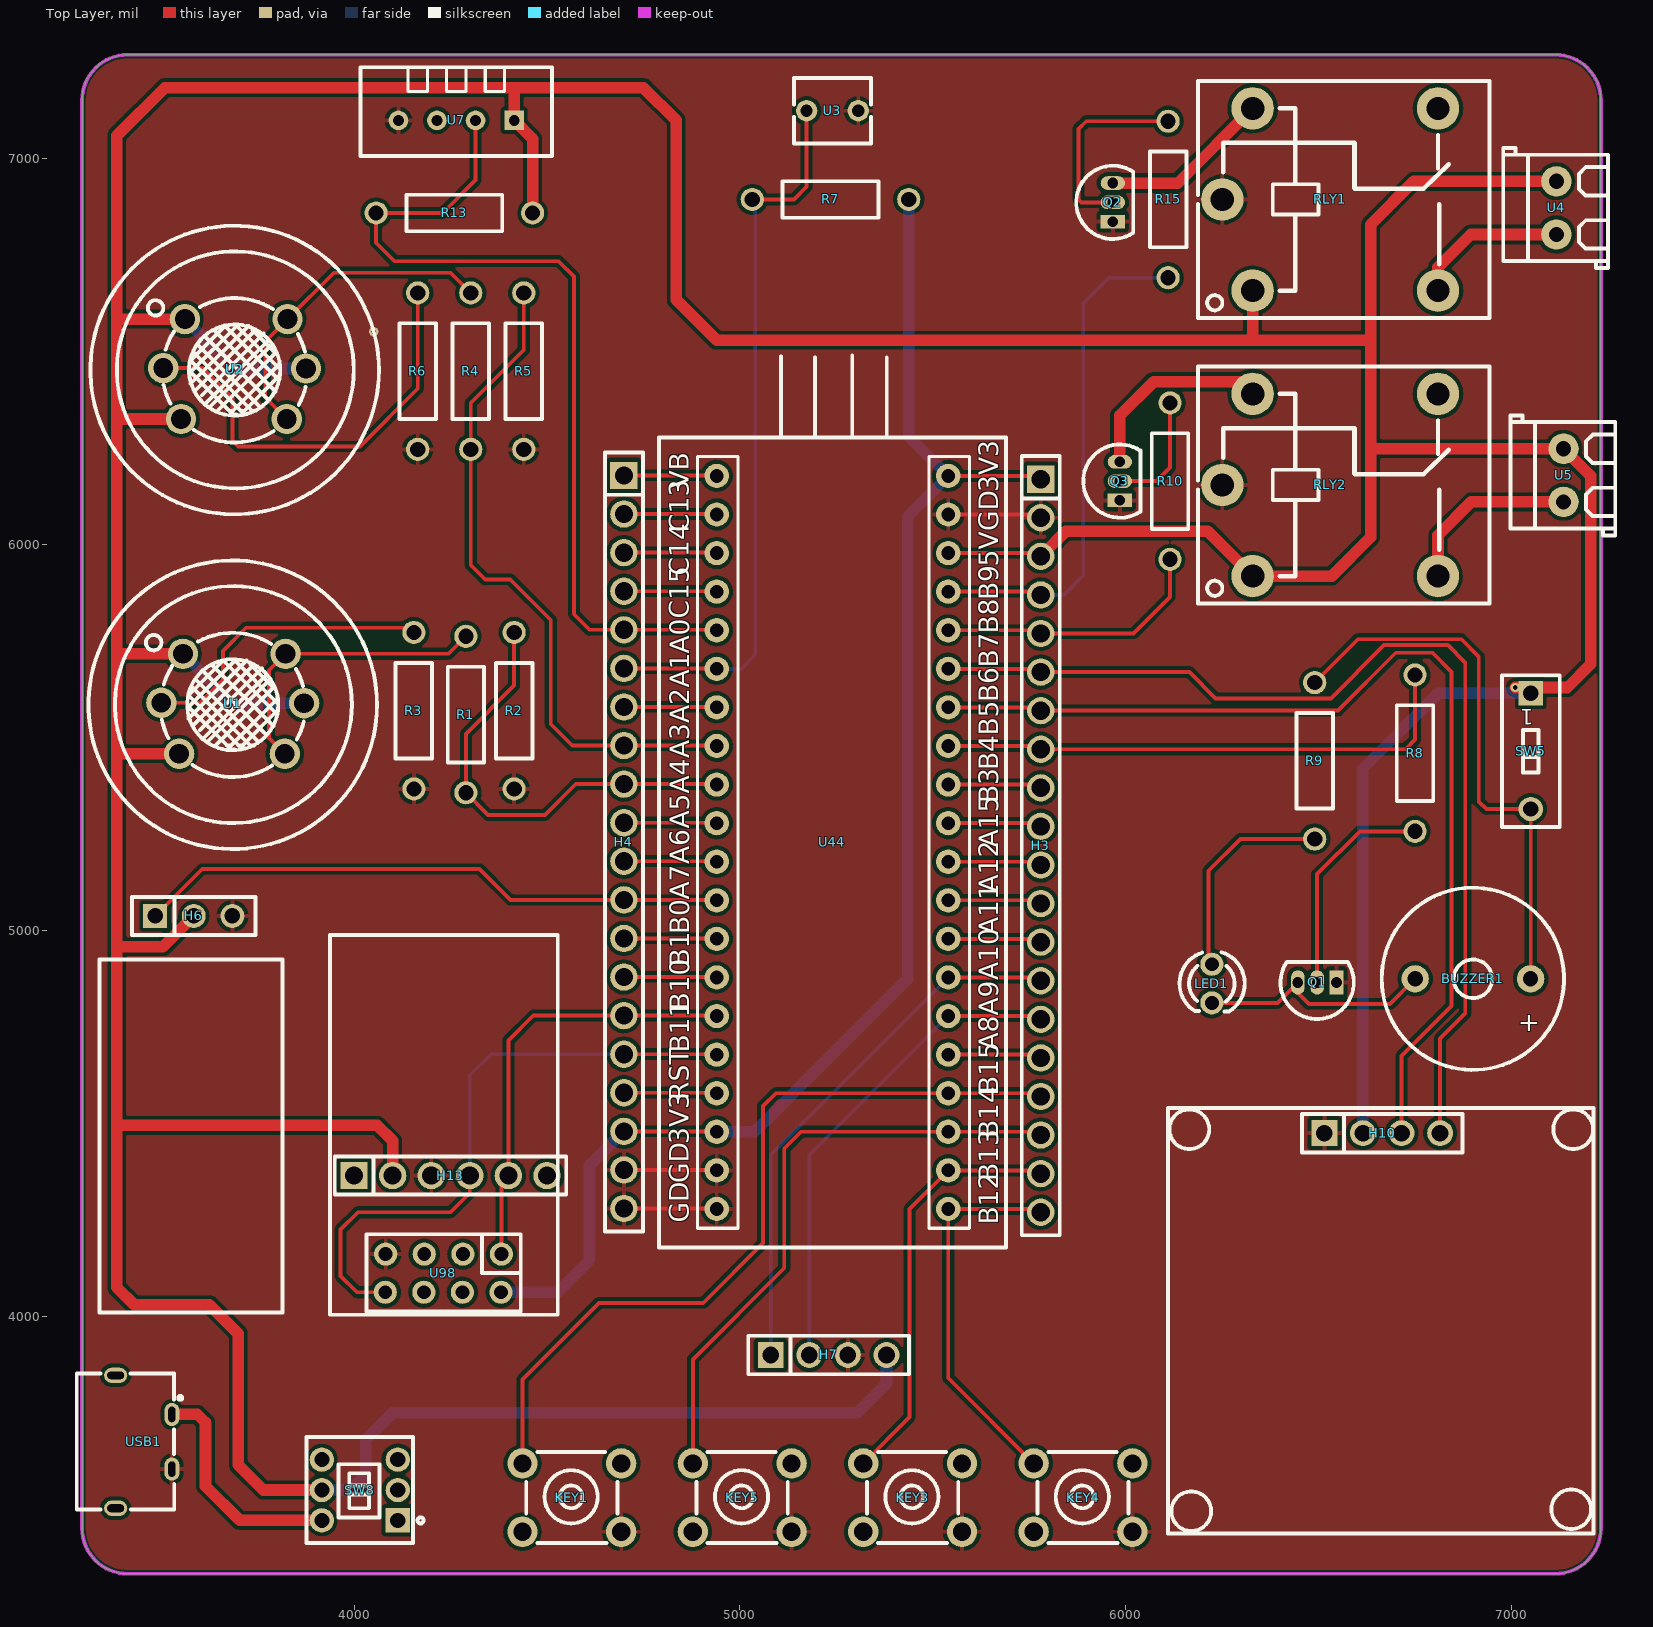
[diagram p0: Top Layer view]
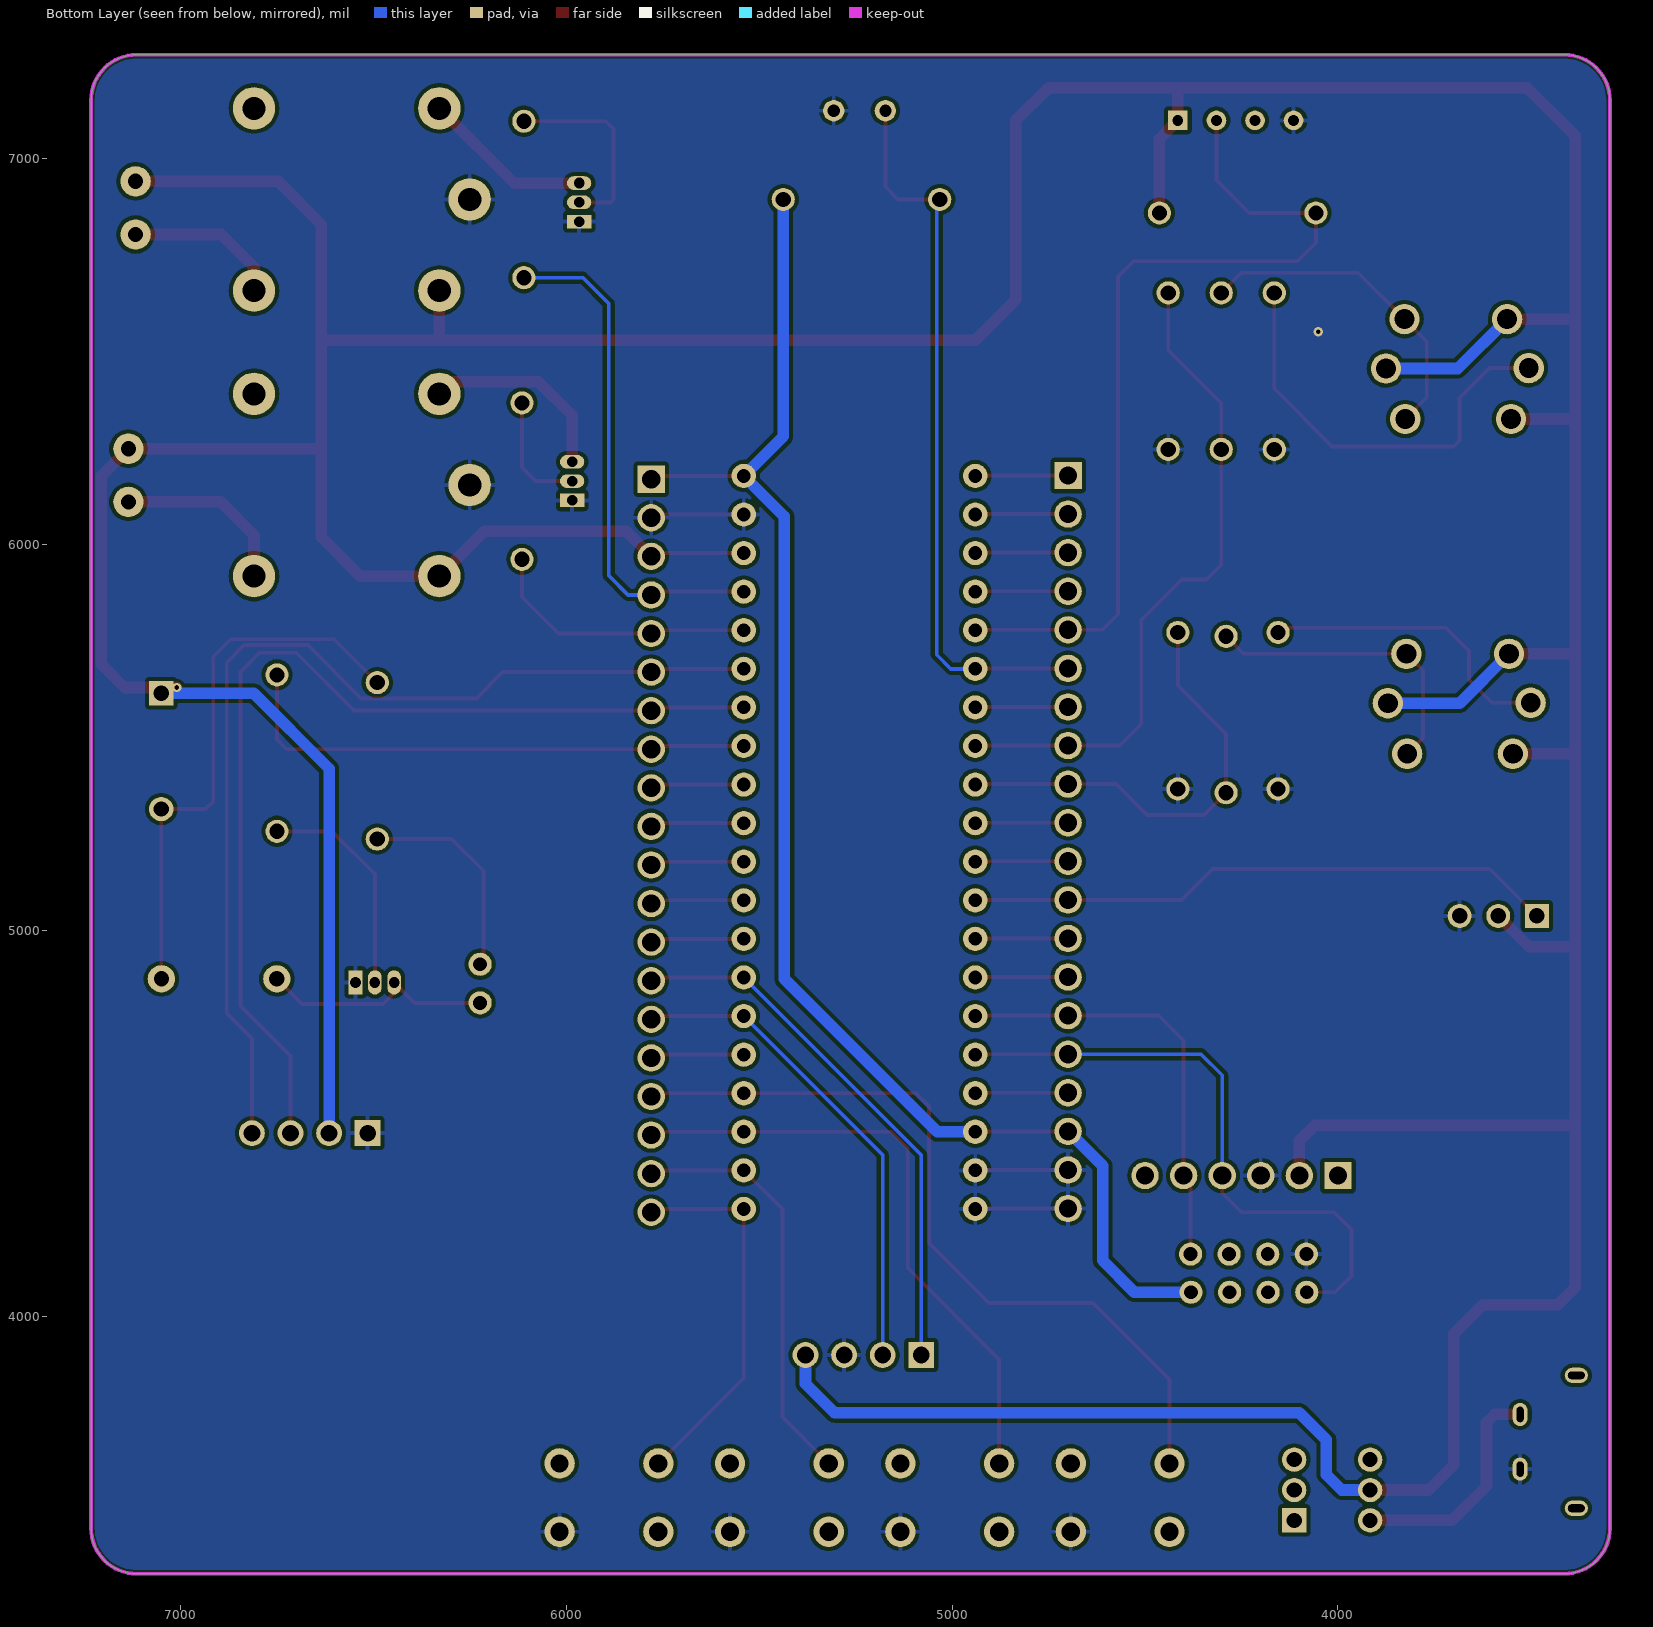
[diagram p1: Bottom Layer view, seen from below]
# Altium PCB MISC62290.pcbdoc
Units mil, origin at the board's own origin, x right, y up, seen from the top; angles counter-clockwise.
Board outline 3937.01 x 3937.01 mil, 2 copper layers (Top Layer, Bottom Layer), stack 62.206 mil thick; 40 components, 52 nets, 202 pads, 2 vias.

## Layer stack, top to bottom
Top Solder Mask Layer: solder mask 0.394, Dk 3.3
Top Layer: signal copper 1.379
Dielectric1: surface 59.449, FR4, Dk 4.5
Bottom Layer: signal copper 1.378
Bottom Solder Mask Layer: solder mask 0.394, Dk 3.3

## Board outline
3413.11,7270 ccw(c3413.11,7151.89) 3295,7151.89 3295,3451.1 ccw(c3413.11,3451.1) 3413.11,3332.99 7113.9,3332.99 ccw(c7113.9,3451.1) 7232.01,3451.1 7232.01,7151.89 ccw(c7113.9,7151.89) 7113.9,7270

## Design rules (kind name [scope] priority, off if disabled: settings)
BoardOutlineClearance copperThickness2oz_1 [All] p2 off: genericclearance=7.99 ignorepadtopadclearanceinfootprint=FALSE except(0: Arc-SplitContinuation Track-SplitContinuation SMDPad-SplitContinuation THPad-SplitContinuation Via-SplitContinuation Fill-SplitContinuation Region-SplitContinuation Poly-SplitContinuation Text-SplitContinuation Hole-SplitContinuation; 5.98: Arc-CutoutEdge SMDPad-CutoutEdge THPad-CutoutEdge Via-CutoutEdge Fill-CutoutEdge Region-CutoutEdge Text-CutoutEdge; 6.93: Hole-OutlineEdge Hole-CutoutEdge; 10: Poly-OutlineEdge Poly-CutoutEdge; 11.81: Arc-OutlineEdge Track-OutlineEdge SMDPad-OutlineEdge THPad-OutlineEdge Via-OutlineEdge Fill-OutlineEdge Region-OutlineEdge Text-OutlineEdge Track-CutoutEdge)
BoardOutlineClearance copperThickness1oz_1 [All] p4: genericclearance=4.02 ignorepadtopadclearanceinfootprint=FALSE except(0: Arc-SplitContinuation Track-SplitContinuation SMDPad-SplitContinuation THPad-SplitContinuation Via-SplitContinuation Fill-SplitContinuation Region-SplitContinuation Poly-SplitContinuation Text-SplitContinuation Hole-SplitContinuation; 6: SMDPad-CutoutEdge THPad-CutoutEdge Via-CutoutEdge Fill-CutoutEdge Region-CutoutEdge Text-CutoutEdge; 6.93: Hole-OutlineEdge Hole-CutoutEdge; 10: Poly-OutlineEdge Poly-CutoutEdge; 11.8: Arc-OutlineEdge Track-OutlineEdge SMDPad-OutlineEdge THPad-OutlineEdge Via-OutlineEdge Fill-OutlineEdge Region-OutlineEdge Text-OutlineEdge; 11.81: Arc-CutoutEdge Track-CutoutEdge)
Clearance copperThickness2oz [All] p1 off: gap=7.99 ignorepadtopadclearanceinfootprint=FALSE except(5.98: SMDPad-Track SMDPad-SMDPad THPad-Track SMDPad-THPad THPad-THPad Track-Via SMDPad-Via THPad-Via Via-Via Fill-Track Region-Track Fill-SMDPad Region-SMDPad Fill-THPad Region-THPad Fill-Via Region-Via Fill-Fill Fill-Region Region-Region Arc-Track Arc-SMDPad Arc-THPad Arc-Via Fill-Arc Region-Arc Arc-Arc Text-Track SMDPad-Text Text-THPad Text-Via Fill-Text Region-Text Arc-Text Text-Text; 6.93: Hole-Track Hole-SMDPad Hole-THPad Hole-Via Fill-Hole Region-Hole Hole-Arc Hole-Text; 10: Poly-Track Poly-SMDPad Poly-THPad Poly-Via Poly-Fill Poly-Region Poly-Poly Poly-Arc Poly-Text Poly-Hole)
Clearance copperThickness1oz [All] p3: gap=4.02 ignorepadtopadclearanceinfootprint=FALSE except(5.98: SMDPad-Track SMDPad-SMDPad THPad-Track SMDPad-THPad THPad-THPad Track-Via SMDPad-Via THPad-Via Via-Via Fill-Track Region-Track Fill-SMDPad Region-SMDPad Fill-THPad Region-THPad Fill-Via Region-Via Fill-Fill Fill-Region Region-Region; 6: Arc-Track Arc-SMDPad Arc-THPad Arc-Via Fill-Arc Region-Arc Arc-Arc Text-Track SMDPad-Text Text-THPad Text-Via Fill-Text Region-Text Arc-Text Text-Text; 6.93: Hole-Track Hole-SMDPad Hole-THPad Hole-Via Fill-Hole Region-Hole Hole-Arc Hole-Text; 10: Poly-Track Poly-SMDPad Poly-THPad Poly-Via Poly-Fill Poly-Region Poly-Poly Poly-Arc Poly-Text Poly-Hole)
Creepage creepage [All] p1: checkdistance=0 ignoreinternallayers=TRUE applytopolygonpour=TRUE
DiffPairsRouting differentialPair [All] p1: maxlimit=6 minlimit=6 mostfreqgap=6 toplayer_minwidth=5 toplayer_prefwidth=10 toplayer_maxwidth=100 toplayer_mingap=6 toplayer_prefgap=6 toplayer_maxgap=6 bottomlayer_minwidth=5 bottomlayer_prefwidth=10 bottomlayer_maxwidth=100 bottomlayer_mingap=6 bottomlayer_prefgap=6 bottomlayer_maxgap=6 maxuncoupledlength=10
HoleToHoleClearance otherClearance [All] p1: gap=11.81 allowstackedmicrovias=TRUE
Length netLength [All] p1: minlimit=0 maxlimit=0
MatchedLengths netLengthTolerance [All] p1: tolerance=1000
PasteMaskExpansion pasteMaskExpansion [All] p1: expansion=0
PlaneConnect innerPlane [All] p1: planeconnectstyle=Relief reliefexpansion=20 reliefentries=4 reliefconductorwidth=10 reliefairgap=10
PolygonConnect copperRegion [(InNet('GND'))] p1: connectstyle=Relief reliefconductorwidth=10 reliefentries=4 polygonreliefangle="90 Angle" airgapwidth=10 via.connectstyle=Relief via.reliefconductorwidth=10 via.reliefentries=4 via.polygonreliefangle="90 Angle" via.airgapwidth=10
RoutingVias viaSize [All] p1: holewidth=12.01 width=24.02 viastyle="Through Hole" minholewidth=11.81 minwidth=19.68 maxholewidth=248.03 maxwidth=393.7
SolderMaskExpansion solderMaskExpansion [IsVia] p1: expansion=-1000 istentingtop=TRUE
SolderMaskExpansion solderMaskExpansion [All] p2: expansion=2 istentingtop=FALSE
Width copperThickness2oz_2 [All] p1 off: maxlimit=100 minlimit=8 preferedwidth=10
Width copperThickness1oz_2 [All] p2: maxlimit=100 minlimit=5 preferedwidth=10

## Components (designator, comment, footprint, x,y, rotation, side; value= is the part's Value field where it differs from the comment)
BUZZER1 "2.3kHz" BUZ-TH_BD12.0-P7.60-D0.6-FD 6900,4875 r180 top
H3 "" HDR-TH_20P-P2.54-V-F 5780,5220 r270 top
H4 "" HDR-TH_20P-P2.54-V-F 4699.46,5229.58 r270 top
H6 "" HDR-TH_3P-P2.54-V-F 3584.58,5037.88 r0 top
H7 "" HDR-TH_4P-P2.54-V-F 5230,3900 r0 top
H10 "2.54-1*4P female" HDR-TH_4P-P2.54-V-F 6665,4475 r0 top
H13 "" HDR-TH_6P-P2.54-V-M-1 4250,4365 r0 top
KEY1 "Button 1" KEY-TH_4P-L6.0-W6.0-P4.50-LS7.5 4564.46,3530.41 r0 top
KEY3 "Button 2" KEY-TH_4P-L6.0-W6.0-P4.50-LS7.5 5447.8,3530.41 r0 top
KEY4 "Button 4" KEY-TH_4P-L6.0-W6.0-P4.50-LS7.5 5889.46,3530.41 r0 top
KEY5 "Button 5" KEY-TH_4P-L6.0-W6.0-P4.50-LS7.5 5006.13,3530.41 r0 top
LED1 "" LED_TH-3mm 6223.5,4862.73 r270 top
Q1 "" S8050_TO_92 6496.32,4865.58 r180 top
Q2 "" S8050_TO_92 5966.77,6887.54 r90 top
Q3 "" S8050_TO_92 5985,6165 r90 top
R1 "10kΩ" Res_1/4W 4290,5560 r90 top
R2 "10kΩ" Res_1/4W 4415,5570 r90 top
R3 "5Ω" Res_1/4W 4155,5570 r90 top
R4 "10kΩ" Res_1/4W 4302.5,6450 r90 top
R5 "10kΩ" Res_1/4W 4440,6450 r90 top
R6 "5Ω" Res_1/4W 4165,6450 r90 top
R7 "1kΩ" Res_1/4W 5235,6895 r180 top
R8 "1kΩ" Res_1/4W 6750,5460 r270 top
R9 "120" Res_1/4W 6490,5440 r270 top
R10 "1kΩ" Res_1/4W 6115,6165 r90 top
R13 "10kΩ" Res_1/4W 4260,6860 r0 top
R15 "1kΩ" Res_1/4W 6110,6895 r90 top
RLY1 "SRD-05VDC-SL-C" RELAY-TH_SRD-XXVDC-XL-C 6530,6895 r0 top
RLY2 "SRD-05VDC-SL-C" RELAY-TH_SRD-XXVDC-XL-C 6530,6155 r0 top
SW5 "NDS-01V" SW-TH_2P-L3.9-W9.9-P2.54-LS7.6 7050,5465 r270 top
SW8 "TK-6700-1" SW-TH_TK-6700-1 4015,3550 r90 top
U1 "MQ-2" SENSOR-TH_MQ-2 3685.58,5587.88 r0 top
U2 "MQ-5" SENSOR-TH_MQ-2 3690.58,6455.41 r0 top
U3 "光敏电阻-5MM" RES-TH_L4.9-W4.3-P3.4 5240,7125 r180 top
U4 "KF350-3.5-2P" CONN-TH_P3.50_KF350-3.5-2P 7116.51,6873.11 r90 top
U5 "KF350-3.5-2P" CONN-TH_P3.50_KF350-3.5-2P 7135,6180 r90 top
U7 "DHT11" SENSOR-TH_DHT11 4265,7100 r180 top
U44 "" STM32最小系统板 5280,5485 r0 top
U98 "" WiFi封装 4230,4370 r0 top
USB1 "KH-TYPE-C-2P" USB-SMD_KH-TYPE-C-2P 3455,3675 r270 top

## Footprints (in the part's own frame and the unit in brackets; to place one, negate y for a bottom-side part, rotate by r counter-clockwise, add the part's x,y. Pads: shape width x height; smd on the part's side, far side on the other; paste and mask are expansions set on the pad)
BUZ-TH_BD12.0-P7.60-D0.6-FD [mm]
  round 1.8 hole 1 paste+0 mask+0.051: 1(-3.8,0) 2(3.8,0)
  silkscreen extent -6,-6 6,6
CONN-TH_P3.50_KF350-3.5-2P [mm]
  round 2 hole 1: 1(-1.75,0) 2(1.75,0)
  silkscreen extent -3.95,-3.4 3.95,3.5
HDR-TH_3P-P2.54-V-F [mil]
  rect 62x62 hole 40.16: 1(-100,0)
  round 62 hole 40.16: 2(0,0) 3(100,0)
  silkscreen extent -160,-49 160,49
HDR-TH_4P-P2.54-V-F [mm]
  rect 1.7x1.7 hole 1.1: 1(-3.81,0)
  round 1.7 hole 1.1: 2(-1.27,0) 3(1.27,0) 4(3.81,0)
  silkscreen extent -5.29,-1.27 5.29,1.27
HDR-TH_6P-P2.54-V-M-1 [mm]
  rect 1.8x1.8 hole 1.2: 1(-6.35,0)
  round 1.8 hole 1.2: 2(-3.81,0) 3(-1.27,0) 4(1.27,0) 5(3.81,0) 6(6.35,0)
  silkscreen extent -7.62,-1.25 7.62,1.25
HDR-TH_20P-P2.54-V-F [mm]
  rect 1.8x1.8 hole 1.2: 1(-24.13,0)
  round 1.8 hole 1.2: 2(-21.59,0) 3(-19.05,0) 4(-16.51,0) 5(-13.97,0) 6(-11.43,0) 7(-8.89,0) 8(-6.35,0) 9(-3.81,0) 10(-1.27,0) 11(1.27,0) 12(3.81,0) 13(6.35,0) 14(8.89,0) 15(11.43,0) 16(13.97,0) 17(16.51,0) 18(19.05,0) 19(21.59,0) 20(24.13,0)
  silkscreen extent -25.65,-1.25 25.65,1.25
KEY-TH_4P-L6.0-W6.0-P4.50-LS7.5 [mm]
  round 2 hole 1.2 paste+0 mask+0.051: 1(-3.25,-2.25) 2(3.25,-2.25) 3(3.25,2.25) 4(-3.25,2.25)
  silkscreen extent -3,-3 3,3
LED_TH-3mm [mil]
  round 60 hole 36 paste+0 mask+2: 1(-50,0) 2(50,0)
  silkscreen extent -81,-84 72,85
RELAY-TH_SRD-XXVDC-XL-C [mil]
  round 110 hole 60: 1(-200.79,-236.22) 2(279.52,-236.2) 3(279.53,236.2) 4(-200.79,236.22) 5(-279.53,0)
  silkscreen extent -342,-307 413,307
RES-TH_L4.9-W4.3-P3.4 [mm]
  round 1.4 hole 0.8 paste+0 mask+0.05: 1(-1.7,0) 2(1.7,0)
  silkscreen extent -2.54,-2.16 2.54,2.16
Res_1/4W [mil]
  round 60 hole 39.37 paste+0 mask+2: 1(-202.76,0) 2(202.76,0)
  silkscreen extent -124,-47 124,47
S8050_TO_92 [mil]
  rect 35.4x63 hole 27.6 paste+0 mask+2: 1(-50,0)
  oval 35.4x63 hole 27.6 paste+0 mask+2: 2(0,0) 3(50,0)
  silkscreen extent -95,-53 95,95
SENSOR-TH_DHT11 [mil]
  rect 51x51 hole 28: 1(-150,0)
  round 51 hole 28: 2(-50,0) 3(50,0) 4(150,0)
  silkscreen extent -248,-138 248,93
SENSOR-TH_MQ-2 [mil]
  round 78.74 hole 51.18: 1(-129,129.5) 2(-185,2.5) 3(-139,-129.5) 4(135,-129.5) 5(185,1.5) 6(137,129.5)
  silkscreen extent -374,-376 374,371
STM32最小系统板 [mm]
  round 1.6 hole 0.9: 1(-8.634,17.614) 2(-8.634,15.074) 3(-8.634,12.534) 4(-8.634,9.994) 5(-8.634,7.454) 6(-8.634,4.914) 7(-8.634,2.374) 8(-8.634,-0.166) 9(-8.634,-2.706) 10(-8.634,-5.246) 11(-8.634,-7.786) 12(-8.634,-10.326) 13(-8.634,-12.866) 14(-8.634,-15.406) 15(-8.634,-17.946) 16(-8.634,-20.486) 17(-8.634,-23.026) 18(-8.634,-25.566) 19(-8.634,-28.106) 20(-8.634,-30.646) 21(6.606,17.614) 22(6.606,15.074) 23(6.606,12.534) 24(6.606,9.994) 25(6.606,7.454) 26(6.606,4.914) 27(6.606,2.374) 28(6.606,-0.166) 29(6.606,-2.706) 30(6.606,-5.246) 31(6.606,-7.786) 32(6.606,-10.326) 33(6.606,-12.866) 34(6.606,-15.406) 35(6.606,-17.946) 36(6.606,-20.486) 37(6.606,-23.026) 38(6.606,-25.566) 39(6.606,-28.106) 40(6.606,-30.646)
  silkscreen extent -12.44,-33.19 10.42,25.54
SW-TH_2P-L3.9-W9.9-P2.54-LS7.6 [mm]
  rect 1.6x1.6 hole 1 paste+0 mask+0.05: 1(-3.81,0)
  round 1.6 hole 1 paste+0 mask+0.05: 2(3.81,0)
  silkscreen extent -5,-1.91 5,1.91
SW-TH_TK-6700-1 [mm]
  rect 1.6x1.6 hole 1 paste+0 mask+0.051: 1(-2,-2.5)
  round 1.6 hole 1 paste+0 mask+0.051: 2(0,-2.5) 3(2,-2.5)
  round 1.6 hole 1 copper offset 0,0 paste+0 mask+0.051: 4(-2,2.5) 5(0,2.5) 6(2,2.5)
  silkscreen extent -3.5,-4.2 3.5,3.5
USB-SMD_KH-TYPE-C-2P [mm]
  oval 1.524x1 hole 0.45 slot 1 at 0 deg paste+0 mask+0.05: 1(-1.8,1.85) 2(1.8,1.85)
  oval 1x1.524 hole 0.5 slot 1.1 at 90 deg paste+0 mask+0.05: 3(4.375,-1.85) 4(-4.375,-1.85)
  silkscreen extent -4.5,-4.41 4.46,2.53
WiFi封装 [mil]
  round 60 hole 36: 1(152.01,-208.54) 2(150.91,-307.4) 3(52.01,-208.54) 4(50.91,-307.4) 5(-47.99,-208.54) 6(-49.09,-307.4) 7(-147.99,-208.54) 8(-149.09,-307.4)
  silkscreen extent -293,-366 298,618

## Via types
v1: diameter 24.02, hole 12, Top Layer to Bottom Layer, 2 vias

## Nets (pads, with @x,y where several pads share a name; then routed paths per layer and width w, separated by ;. In a path a pad name is that pad's centre, name@x,y a point inside that pad or via, vN(x,y) a via of type N, cw(c..) or ccw(c..) an arc to the next point about the centre after c; other vN are vias at no path point)
3V3: H3.1 H4.18 R7.1 U44.18 U44.21 U98.2 | length 3895.4
  Top Layer w10: H4.18 U44.18@4940,4479.58 ; U44.21 H3.1@5795,6178.46
  Bottom Layer w30: U98.2 4527.6,4062.6 4610,4145 4610,4390.12 H4.18 ; U44.18 5038.46,4478.46 5435,4875 5435,6073.39 U44.21 5437.76,6280.78 R7.1
$1N3: R1.2 U1.4 U1.6 | length 779.7
  Top Layer w10: U1.4 3780,5498.95 3780,5674.8 U1.6 4244.61,5717.38 R1.2
$1N5: R3.2 U1.2 | length 784
  Top Layer w10: U1.2 3600.38,5590.38 3660,5650 3660,5725 3720,5785 4142.76,5785 R3.2
$1N8: R6.2 U2.2 | length 1117.8
  Top Layer w10: U2.2 3607.09,6457.91 3685,6380 3685,6270 3700,6255 4015,6255 4165,6405 R6.2
$1N10: R4.2 U2.4 U2.6 | length 852.2
  Top Layer w10: U2.4 3770,6381.49 3770,6527.33 U2.6 3947.67,6705 4250.26,6705 R4.2
$1N88: BUZZER1.1 R9.1 SW5.2 | length 1448.6
  Top Layer w10: R9.1 6602.24,5755 6870,5755 6915,5710 6915,5335 6935,5315 SW5.2 7050,4875.4 BUZZER1.1
$1N89: BUZZER1.2 LED1.2 Q1.3 | length 614.5
  Top Layer w10: LED1.2 6393.47,4812.73 Q1.3 6446.32,4838.68 6475,4810 6685.4,4810 BUZZER1.2
$1N100: H4.17 U44.17 | length 240.5
  Top Layer w10: H4.17 U44.17@4940,4579.58
$1N103: H4.14 U44.14 | length 240.5
  Top Layer w10: H4.14 U44.14@4940,4879.58
$1N104: H4.13 U44.13 | length 240.5
  Top Layer w10: H4.13 U44.13@4940,4979.58
$1N106: H4.11 U44.11 | length 240.5
  Top Layer w10: H4.11 U44.11@4940,5179.58
$1N110: H4.7 U44.7 | length 240.5
  Top Layer w10: H4.7 U44.7@4940,5579.58
$1N113: H4.4 U44.4 | length 240.5
  Top Layer w10: H4.4 U44.4@4940,5879.58
$1N114: H4.3 U44.3 | length 240.5
  Top Layer w10: H4.3 U44.3@4940,5979.58
$1N115: H4.2 U44.2 | length 240.5
  Top Layer w10: H4.2 U44.2@4940,6079.58
$1N116: H4.1 U44.1 | length 240.5
  Top Layer w10: H4.1 U44.1@4940,6179.58
$1N125: H3.9 U44.29 | length 254.9
  Top Layer w10: U44.29 H3.9@5795,5378.46
$1N126: H3.10 U44.30 | length 254.9
  Top Layer w10: U44.30 H3.10@5795,5278.46
$1N127: H3.11 U44.31 | length 254.9
  Top Layer w10: U44.31 H3.11@5795,5178.46
$1N128: H3.12 U44.32 | length 254.9
  Top Layer w10: U44.32 H3.12@5795,5078.46
$1N129: H3.13 U44.33 | length 254.9
  Top Layer w10: U44.33 H3.13@5795,4978.46
$1N132: H3.16 U44.36 | length 254.9
  Top Layer w10: U44.36 H3.16@5795,4678.46
$1N154: RLY1.2 U4.1 | length 402.8
  Top Layer w30: RLY1.2 6809.53,6719.53 6894.21,6804.21 U4.1
$1N275: Q1.2 R8.2 | length 580.4
  Top Layer w10: Q1.2 6496.32,5146.32 6607.24,5257.24 R8.2
$1N288: Q2.2 R15.2 | length 515.4
  Top Layer w10: Q2.2 5885,6887.54 5877.93,6894.61 5877.93,7077.93 5897.76,7097.76 R15.2
$1N290: Q2.3 RLY1.4 | length 442.7
  Top Layer w30: Q2.3 6135.53,6937.54 RLY1.4
$1N291: Q3.3 RLY2.4 | length 513.6
  Top Layer w30: Q3.3 5985,6335.21 6072.38,6422.59 6297.84,6422.59 RLY2.4
$1N293: Q3.2 R10.2 | length 312.3
  Top Layer w10: Q3.2 6080,6165 6115,6200 R10.2
$1N298: RLY2.2 U5.1 | length 467.1
  Top Layer w30: RLY2.2 6809.53,6024.53 6896.1,6111.1 U5.1
$1N299: LED1.1 R9.2 | length 554.9
  Top Layer w10: LED1.1 6215,4921.24 6215,5155 6297.24,5237.24 R9.2
+5V: H3.3 H6.2 H7.4 H10.2 H13.2 R13.2 RLY1.1 RLY2.1 SW5.1 SW8.5 U1.1 U1.3 U1.5 U2.1 U2.3 U2.5 U4.2 U5.2 U7.1 U44.23 | length 17757.5
  Top Layer w10: U44.23 H3.3@5788.46,5978.46
  Top Layer w30: 3385.03,5717.38 U1.1 ; U1.3 3388.56,5458.38 3385,5461.93 ; U2.3 3388.18,6325.91 3385,6329.09 ; U2.1 3387.29,6584.91 3385,6587.2 ; H6.2 3504.66,4957.95 3385,4957.95 ; SW8.5 3765,3550 3700,3615 3700,3955 3625,4030 3430,4030 3385,4075 3385,4490.1 ; H13.2 4100,4455 4060,4495 3389.9,4495 3385,4490.1 ; R13.2 4462.76,7052.24 U7.1 4415,7183.35 4416.65,7185 ; H3.3 5788.46,5978.46 5845,6035 6212.99,6035 RLY2.1 6533.78,5918.78 6635,6020 6635,6254.11 ; RLY1.1 6329.21,6530.46 6328.75,6530 ; v1(7010,5630) 7145,5630 7205,5690 7205,6178.9 U5.2 6640.22,6248.9 6635,6254.11 ; U4.2 6747,6942 6635,6830 6635,6530 ; 3385,4490.1 3385,4957.95 ; 3385,4957.95 3385,5461.93 ; 3385,5461.93 3385,5717.41 3385,6329.09 ; 3385,6329.09 3385,6587.2 ; 3385,6587.2 3385,7060 3510,7185 4416.65,7185 ; 4416.65,7185 4750,7185 4835,7100 4835,6635 4940,6530 6328.75,6530 ; 6328.75,6530 6635,6530 ; 6635,6254.11 6635,6530
  Bottom Layer w30: U1.1 3684.58,5589.38 U1.5 ; U2.1 3689.58,6456.91 U2.5 ; SW8.5 3990,3550 4030,3590 4030,3680 4100,3750 5305,3750 5380,3825 H7.4 ; H10.2 6615,5420 6810,5615 SW5.1
GND: H3.2 H4.19 H4.20 H6.3 H7.3 H10.1 H13.3 KEY1.2 KEY3.2 KEY4.2 KEY5.2 Q1.1 Q2.1 Q3.1 R2.1 R3.1 R5.1 R6.1 RLY1.5 RLY2.5 U3.1 U7.4 U44.19 U44.20 U44.22 U98.7 USB1.2 | length 736
  Top Layer w10: H4.20 U44.20@4940,4279.58 ; H4.19 U44.19@4940,4379.58 ; U44.22 H3.2@5795,6078.46
  other v1: 4051.2,6552.12
PA0: H4.5 R13.1 U7.2 U44.5 | length 2336.1
  Top Layer w10: U7.2 4315,6945 4230,6860 R13.1 4057.24,6782.76 4105,6735 4530,6735 4570,6695 4570,5820 4610.42,5779.58 H4.5 U44.5@4940,5779.58
PA1: H4.6 R7.2 U3.2 U44.6 | length 1890.3
  Top Layer w10: H4.6 U44.6@4940,5679.58 ; R7.2 5140,6895 5173.07,6928.07 U3.2
  Bottom Layer w10: U44.6 5003.46,5678.46 5040,5715 5040,6887.24 R7.2
PA3: H4.8 R4.1 R5.2 U44.8 | length 1751.7
  Top Layer w10: R5.2 4440,6505 4302.5,6367.5 R4.1 4302.5,5947.5 4340,5910 4405,5910 4510,5805 4510,5535 4565.42,5479.58 H4.8 U44.8@4940,5479.58
PA4: H4.9 R1.1 R2.2 U44.9 | length 1174
  Top Layer w10: R2.2 4415,5635 4290,5510 R1.1 4347.24,5300 4495,5300 4574.58,5379.58 H4.9 U44.9@4940,5379.58
PA5: H4.10 U44.10 | length 240.5
  Top Layer w10: H4.10 U44.10@4940,5279.58
PA7: H4.12 H6.1 U44.12 | length 1539.3
  Top Layer w10: H6.1 3606.7,5160 4325,5160 4405.42,5079.58 H4.12 U44.12@4940,5079.58
PB5: H3.8 R8.1 U44.28 | length 1403
  Top Layer w10: U44.28 H3.8@5795,5478.46 ; H3.8 6725,5470 6750,5495 R8.1
PB6: H3.7 H10.3 U44.27 | length 2651.6
  Top Layer w10: U44.27 H3.7@5795,5578.46 ; H3.7 6550,5570 6700,5720 6795,5720 6845,5670 6845,4805 6715,4675 H10.3
PB7: H3.6 H10.4 U44.26 | length 2706
  Top Layer w10: U44.26 H3.6@5795,5678.46 ; H3.6 6165,5670 6233.22,5601.78 6531.78,5601.78 6670,5740 6835,5740 6880,5695 6880,4785 6815,4720 H10.4
PB8: H3.5 R10.1 U44.25 | length 726.5
  Top Layer w10: U44.25 H3.5@5795,5778.46 ; H3.5 6020,5770 6115,5865 R10.1
PB9: H3.4 R15.1 U44.24 | length 1338.5
  Top Layer w10: U44.24 H3.4@5795,5878.46
  Bottom Layer w10: H3.4 5840,5870 5890,5920 5890,6625 5957.24,6692.24 R15.1
PB12: H3.20 KEY4.4 U44.40 | length 1006.1
  Top Layer w10: KEY4.4 5540.08,3840.43 U44.40 H3.20@5795,4278.46
PB13: H3.19 KEY3.4 U44.39 | length 1105.6
  Top Layer w10: KEY3.4 5440,3739.14 5440,4278.39 U44.39 H3.19@5795,4378.46
PB14: H3.18 KEY5.4 U44.38 | length 1612.1
  Top Layer w10: KEY5.4 4878.18,3888.18 5115,4125 5115,4435 5158.46,4478.46 U44.38 H3.18@5795,4478.46
PB15: H3.17 KEY1.4 U44.37 | length 2091.3
  Top Layer w10: KEY1.4 4436.51,3836.51 4635,4035 4905,4035 5060,4190 5060,4545 5093.46,4578.46 U44.37 H3.17@5795,4578.46
U1_RX: H3.14 H7.1 U44.34 | length 1424
  Top Layer w10: U44.34 H3.14@5795,4878.46
  Bottom Layer w10: H7.1 5080,4418.39 U44.34
U1_TX: H3.15 H7.2 U44.35 | length 1282.5
  Top Layer w10: U44.35 H3.15@5795,4778.46
  Bottom Layer w10: H7.2 5180,4418.39 U44.35
U3_RX: H4.16 H13.4 U44.16 U98.8 | length 1595.4
  Top Layer w10: U98.8 4007.4,4062.6 3965,4105 3965,4225 4010,4270 4250,4270 4300,4320 H13.4 ; H4.16 U44.16@4940,4679.58
  Bottom Layer w10: H13.4 4300,4625 4354.58,4679.58 H4.16
U3_TX: H4.15 H13.5 U44.15 U98.1 | length 1127.7
  Top Layer w10: U98.1 4382.01,4347.01 H13.5 4400,4715 4464.58,4779.58 H4.15 U44.15@4940,4779.58
VUSB: SW8.4 USB1.1 | length 599.1
  Top Layer w30: USB1.1 3594.13,3745.87 3615,3725 3615,3560 3703.74,3471.26 SW8.4
pads on no net: H13.1 H13.6 KEY1.1 KEY1.3 KEY3.1 KEY3.3 KEY4.1 KEY4.3 KEY5.1 KEY5.3 RLY1.3 RLY2.3 SW8.1 SW8.2 SW8.3 SW8.6 U7.3 U98.3 U98.4 U98.5 U98.6 USB1.3 USB1.4

## Polygon pours and split planes (outlines as drawn)
GND on Bottom Layer (solid, remove dead copper, pour order 2): 3000,7550 3000,3000 7640,3000 7640,7550
GND on Top Layer (solid, remove dead copper, pour order 0): 3110,7440 3110,3130 7615,3130 7615,7440

## Keep-outs
Board Outline Layer:
  the board outline again, w10

## Silkscreen, mask and mechanical layers (free items; w line width, h text height)
Top Silkscreen Layer:
  lines w10: 3340,4010 3340,4925 3815,4925 3815,4010 3340,4010